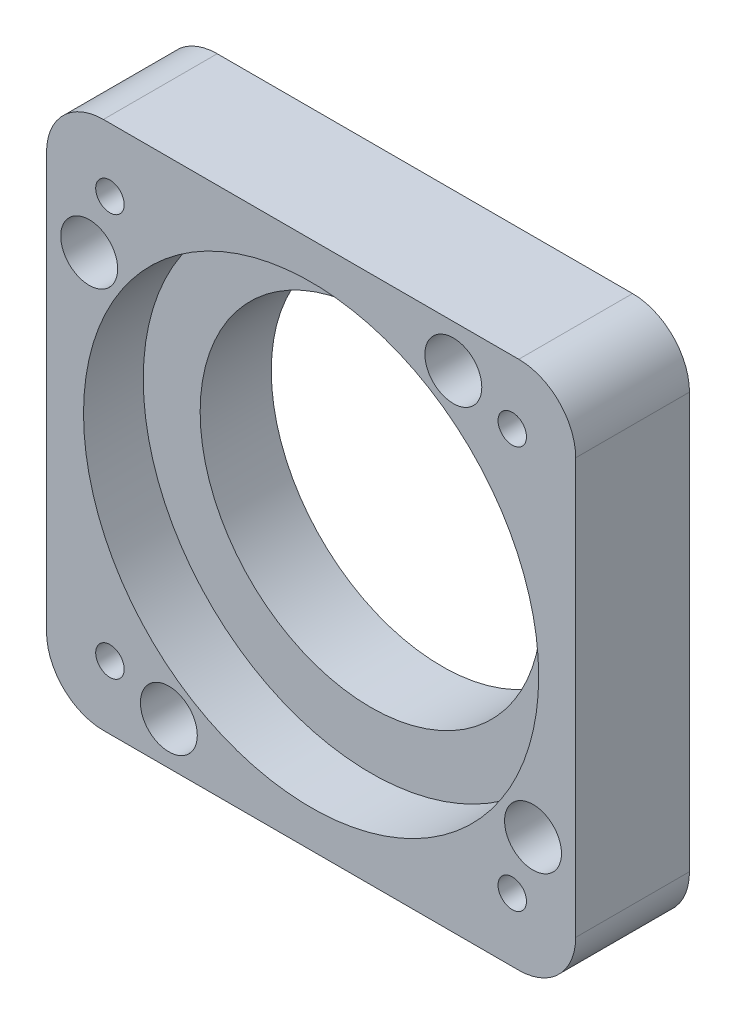
from build123d import *
from build123d.topology import SkipClean

# Parameters (mm, degrees)
SKETCH1_W                                           = 93
SKETCH1_H                                           = 93
SKETCH1_R                                           = 30
BOSS_EXTRUDE1_DEPTH                                 = 20
FILLET1_R                                           = 10
BOSS_EXTRUDE2_START                                 = 3
SKETCH6_R                                           = 41
SKETCH6_R_2                                         = 30
BOSS_EXTRUDE2_DEPTH                                 = 3
SKETCH7_R                                           = 40
CUT_EXTRUDE1_DEPTH                                  = 10.5
M6_TAPPED_HOLE1_D                                   = 5
HOLE_SPEC_PER_SOCKET_HEAD_CAP_SCREW_TYP_D           = 5.5
HOLE_SPEC_PER_SOCKET_HEAD_CAP_SCREW_TYP_CBORE_D     = 10
HOLE_SPEC_PER_SOCKET_HEAD_CAP_SCREW_TYP_CBORE_DEPTH = 9.7
CIRPATTERN2_COUNT                                   = 4


with BuildPart() as part:
    # Sketch1 → Boss-Extrude1 (new body)
    with BuildSketch(Plane.XY):
        Rectangle(SKETCH1_W, SKETCH1_H)
        Circle(SKETCH1_R, mode=Mode.SUBTRACT)
    extrude(amount=BOSS_EXTRUDE1_DEPTH)

    # Fillet1
    fillet1_edges = [part.edges().sort_by_distance(p)[0] for p in [
        (46.5, -46.5, 10),
        (-46.5, -46.5, 10),
        (-46.5, 46.5, 10),
        (46.5, 46.5, 10),
    ]]
    fillet(fillet1_edges, radius=FILLET1_R)

    # Sketch6 → Boss-Extrude2 (add)
    with SkipClean():  # the faces are left unmerged after this step: merging them gives an invalid solid
        with BuildSketch(Plane(origin=(0, 0, 0), x_dir=(-1, 0, 0), z_dir=(0, 0, -1)).offset(BOSS_EXTRUDE2_START)):
            Circle(SKETCH6_R)
            Circle(SKETCH6_R_2, mode=Mode.SUBTRACT)
        extrude(amount=-BOSS_EXTRUDE2_DEPTH)

    # Sketch7 → Cut-Extrude1 (cut)
    with BuildSketch(Plane.XY.offset(20)):
        Circle(SKETCH7_R)
    extrude(amount=-CUT_EXTRUDE1_DEPTH, mode=Mode.SUBTRACT)

    # M6 Tapped Hole1 (through all)
    with Locations(Plane.XY.offset(20)):
        with Locations((-35.355339059, 35.355339059), (35.355339059, 35.355339059), (35.355339059, -35.355339059), (-35.355339059, -35.355339059)):
            Hole(M6_TAPPED_HOLE1_D / 2)

    # Hole Spec (per socket head cap screw type) 1 (through all)
    with Locations(Plane.XY.offset(20)):
        with Locations((-25, -39)):
            hole_spec_per_socket_head_cap_screw_typ = CounterBoreHole(HOLE_SPEC_PER_SOCKET_HEAD_CAP_SCREW_TYP_D / 2, HOLE_SPEC_PER_SOCKET_HEAD_CAP_SCREW_TYP_CBORE_D / 2, HOLE_SPEC_PER_SOCKET_HEAD_CAP_SCREW_TYP_CBORE_DEPTH)

    # CirPattern2: Hole Spec (per socket head cap screw type) 1 ×4 about axis
    cirpattern2_axis = Axis((0, 0, 0), (0, 0, 1))
    for i in range(1, CIRPATTERN2_COUNT):
        add(hole_spec_per_socket_head_cap_screw_typ.rotate(cirpattern2_axis, i * 360 / CIRPATTERN2_COUNT), mode=Mode.SUBTRACT)


solid = part.part
